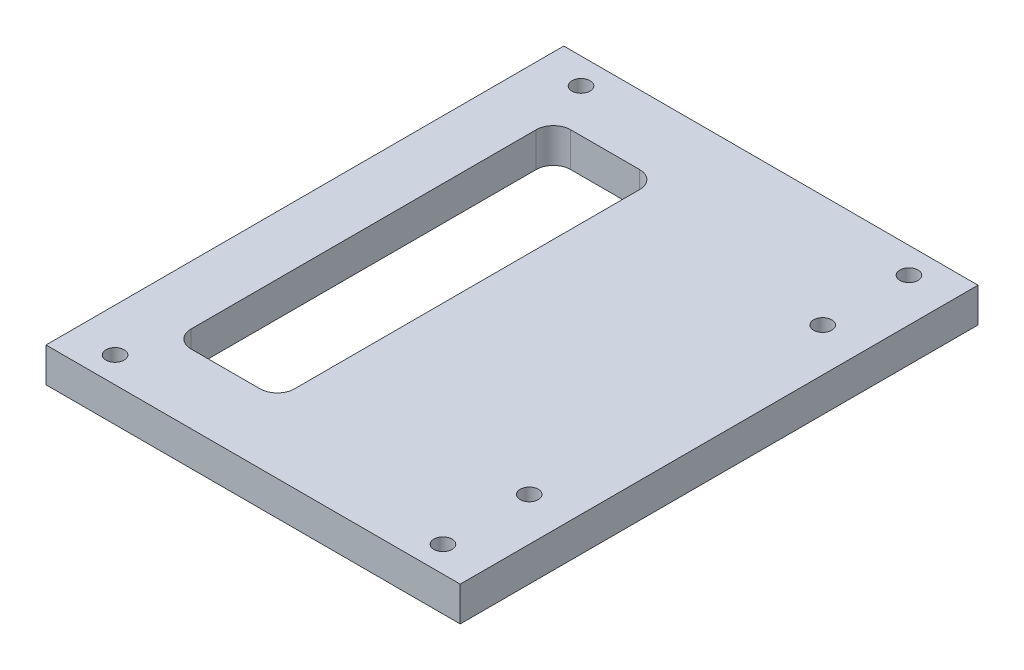
SolidWorks part; units mm, degrees
material "45#"
ref_plane "Front Plane" through (0, 0, 0) normal (0, 0, 1) x (1, 0, 0)
ref_plane "Top Plane" through (0, 0, 0) normal (0, 1, 0) x (1, 0, 0)
ref_plane "Right Plane" through (0, 0, 0) normal (1, 0, 0) x (0, 0, -1)
sketch "Sketch1" plane through (0, 0, 0) normal (0, 1, 0) x (1, 0, 0)
  line L1 (-240, 300) -> (240, 300)
  line L2 (-240, 300) -> (-240, -300)
  line L3 (-240, -300) -> (240, -300)
  line L4 (240, 300) -> (240, -300)
  line L5 (-240, 300) -> (240, -300) construction
  line L6 (-240, -300) -> (240, 300) construction
  point P0 (0, 0)
  dimension "D2" = 600
  dimension "D3" = 480
extrude "Boss-Extrude1" add sketch "Sketch1" along normal blind 40
sketch "Sketch4" plane through (0, 40, 0) normal (0, 1, 0) x (1, 0, 0)
  line L1 (-172, 220) -> (-52, 220)
  line L2 (-172, 220) -> (-172, -220)
  line L3 (-172, -220) -> (-52, -220)
  line L4 (-52, 220) -> (-52, -220)
  line L5 (-172, 220) -> (-52, -220) construction
  line L6 (-172, -220) -> (-52, 220) construction
  line L7 (-240, 300) -> (-240, -300) construction
  line L8 (-240, 0) -> (-172, 0) construction
  dimension "D1" = 120
  dimension "D2" = 440
  dimension "D3" = 68
extrude "Cut-Extrude3" cut sketch "Sketch4" against normal through all
fillet "Fillet1" radius 20 4 edges at (-52, 20, 220) (-172, 20, 220) (-52, 20, -220) (-172, 20, -220)
hole_wizard "M24 Tapped Hole1" positions "Sketch5" profile "Sketch6" tap size "M24" standard "GB" end condition through all
sketch "Sketch5" plane through (0, 40, 0) normal (0, 1, 0) x (1, 0, 0)
  line L0 (0, 0) -> (254.5234, 0) construction
  line L2 (0, 0) -> (0, 93.7338) construction
  line L4 (240, 300) -> (-240, 300) construction
  line L5 (190, 270) -> (190, 170) construction
  point P0 (-190, -270)
  point P8 (-190, 270)
  point P14 (190, 270)
  point P15 (190, -270)
  point P18 (190, 170)
  point P20 (190, -170)
  dimension "D1" = 30
  dimension "D2" = 380
  dimension "D3" = 340
sketch "Sketch6" plane through (-190, 40, 270) normal (1, 0, 0) x (0, 0, 1)
  line L0 (0, 0) -> (0, 40)
  line L1 (0, 40) -> (10.5, 40)
  line L2 (10.5, 40) -> (10.5, 0)
  line L5 (10.5, 0) -> (0, 0)
  line L11 (0, -6.35) -> (0, 107.95) construction
  dimension "通孔螺纹孔钻头直径" = 21
  dimension "通孔螺纹孔钻头深度" = 40
cosmetic thread "Hole Thread1" parameters "D1"=48, "D2"=22
cosmetic thread "Hole Thread2" parameters "D1"=48, "D2"=22
cosmetic thread "Hole Thread3" parameters "D1"=48, "D2"=22
cosmetic thread "Hole Thread4" parameters "D1"=48, "D2"=22
cosmetic thread "Hole Thread5" parameters "D1"=48, "D2"=22
cosmetic thread "Hole Thread6" parameters "D1"=48, "D2"=22
